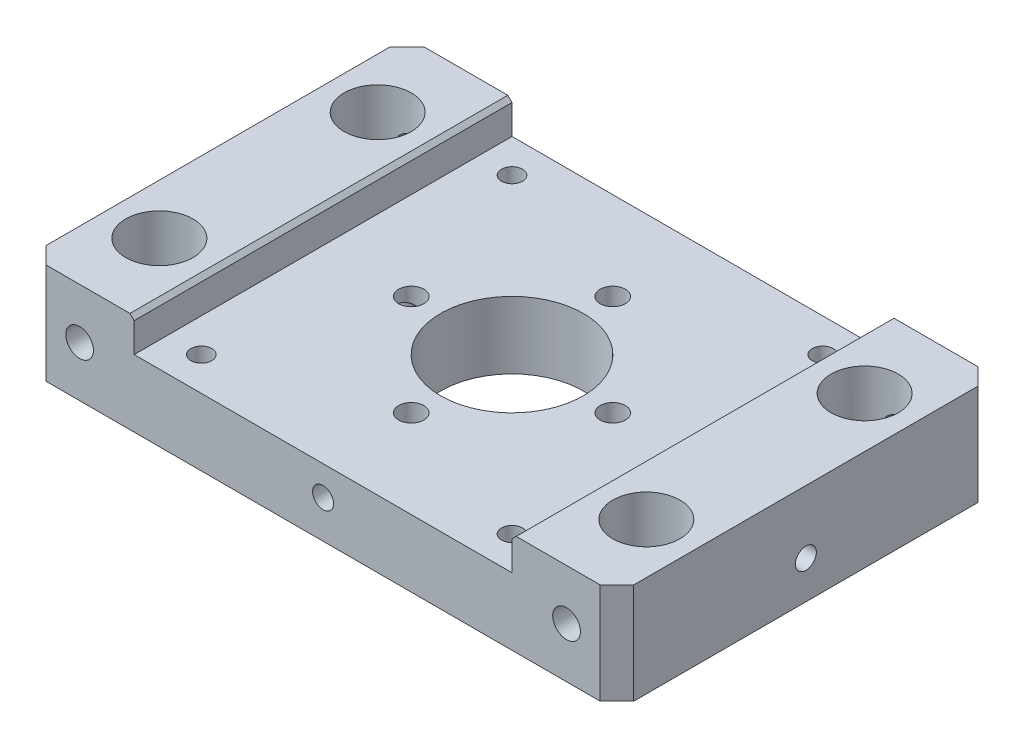
SolidWorks part; units mm, degrees
ref_plane "Front Plane" through (0, 0, 0) normal (0, 0, 1) x (1, 0, 0)
ref_plane "Top Plane" through (0, 0, 0) normal (0, 1, 0) x (1, 0, 0)
ref_plane "Right Plane" through (0, 0, 0) normal (1, 0, 0) x (0, 0, -1)
sketch "Sketch1" plane through (0, 0, 0) normal (0, 1, 0) x (1, 0, 0)
  line L1 (-35, 22.5) -> (35, 22.5)
  line L2 (-35, 22.5) -> (-35, -22.5)
  line L3 (-35, -22.5) -> (35, -22.5)
  line L4 (35, 22.5) -> (35, -22.5)
  line L5 (-35, 22.5) -> (35, -22.5) construction
  line L6 (-35, -22.5) -> (35, 22.5) construction
  point P0 (0, 0)
  dimension "D1" = 45
  dimension "D2" = 70
extrude "Boss-Extrude1" add sketch "Sketch1" along normal blind 12
sketch "Sketch2" plane through (0, 12, 0) normal (0, 1, 0) x (1, 0, 0)
  line L0 (35, 22.5) -> (-35, 22.5) construction
  line L1 (-22.5, -22.5) -> (22.5, -22.5)
  line L2 (-22.5, -22.5) -> (-22.5, 22.5)
  line L3 (-22.5, 22.5) -> (22.5, 22.5)
  line L4 (22.5, -22.5) -> (22.5, 22.5)
  line L5 (-22.5, -22.5) -> (22.5, 22.5) construction
  line L6 (-22.5, 22.5) -> (22.5, -22.5) construction
  point P0 (0, 0)
  dimension "D1" = 45
extrude "Cut-Extrude1" cut sketch "Sketch2" against normal blind 4
sketch "Sketch3" plane through (0, 12, 0) normal (0, 1, 0) x (1, 0, 0)
  line L0 (0, 0) -> (50000, 0) construction
  line L1 (0, 0) -> (0, -50000) construction
  circle A0 centre (-29, 13) radius 4
  circle A1 centre (-29, -13) radius 4
  circle A2 centre (29, -13) radius 4
  circle A3 centre (29, 13) radius 4
  dimension "D2" = 26
  dimension "D3" = 8
  dimension "D1" = 58
extrude "Cut-Extrude2" cut sketch "Sketch3" against normal blind 50
sketch "Sketch4" plane through (0, 12, 0) normal (0, 1, 0) x (1, 0, 0)
  circle A0 centre (0, 0) radius 8.5
  dimension "D1" = 17
extrude "Cut-Extrude3" cut sketch "Sketch4" against normal blind 50
sketch "Sketch5" plane through (0, 0, 22.5) normal (0, 0, 1) x (1, 0, 0)
  line L0 (0, 0) -> (0, -50000) construction
  line L1 (-35, 6) -> (49965, 6) construction
  line L2 (-35, 12) -> (-35, 0) construction
  line L3 (-29, 0) -> (-29, 50000) construction
  line L4 (-35, 12) -> (-22.5, 12) construction
  line L8 (-25, 0) -> (-25, 12) construction
  line L9 (-33, 12) -> (-33, 0) construction
  circle A0 centre (-29, 6) radius 0.5
  circle A1 centre (29, 6) radius 0.5
  point P7 (-35, 6)
  dimension "D1" = 1
extrude "Cut-Extrude4" cut sketch "Sketch5" against normal blind 7
hole_wizard "M4 Tapped Hole1" positions "3DSketch1" profile "Sketch6" tap size "M4" standard "Gb"
sketch3d "3DSketch1"
  line L0 (-29, 6, 17) -> (-29, 6, 22.5) construction
  line L1 (29, 6, 17) -> (29, 6, 22.5) construction
  point P0 (-29, 6, 22.5)
  point P4 (29, 6, 22.5)
sketch "Sketch6" plane through (-29, 6, 22.5) normal (1, 0, 0) x (0, -1, 0)
  line L0 (0, 0) -> (0, 11.0914)
  line L1 (0, 11.0914) -> (1.65, 10.1)
  line L2 (1.65, 10.1) -> (1.65, 0)
  line L5 (1.65, 0) -> (0, 0)
  line L10 (0, 11.0914) -> (-1.65, 10.1) construction
  line L11 (0, -6.35) -> (0, 107.95) construction
  dimension "螺纹孔钻头直径" = 3.3
  dimension "螺纹孔钻头深度" = 10.1
  dimension "导头角度" = 118
cosmetic thread "Hole thread1" parameters "D1"=5.8562, "D2"=4
cosmetic thread "Hole thread2" parameters "D1"=5.8562, "D2"=4
mirror "Mirror1" about plane through (0, 0, 0) normal (0, 0, 1) of "M4 Tapped Hole1"
sketch "Sketch7" plane through (0, 8, 0) normal (0, 1, 0) x (1, 0, 0)
  line L0 (0, 0) -> (50000, 0) construction
  line L1 (0, 0) -> (0, -50000) construction
  circle A0 centre (0, 0) radius 12 construction
  circle A1 centre (0, 12) radius 1.5
  circle A2 centre (12, 0) radius 1.5
  circle A3 centre (0, -12) radius 1.5
  circle A4 centre (-12, 0) radius 1.5
  dimension "D1" = 24
  dimension "D2" = 3
extrude "Cut-Extrude5" cut sketch "Sketch7" against normal blind 4.8
sketch "Sketch8" plane through (-35, 0, 0) normal (-1, 0, 0) x (0, 0, 1)
  line L0 (0, 0) -> (0, 50000) construction
  line L1 (-22.5, 0) -> (22.5, 0) construction
  circle A0 centre (0, 4.5) radius 1.25
  dimension "D1" = 2.5
  dimension "D2" = 4.5
extrude "Cut-Extrude6" cut sketch "Sketch8" against normal blind 23
cosmetic thread "Hole thread9" parameters "D1"=6, "D2"=3
pattern_circular "CirPattern1" count 4 over 360 about axis through (0, -38, 0) along (0, 1, 0) of "Cut-Extrude6"
cosmetic thread "Hole thread7" parameters "D1"=6, "D2"=3
cosmetic thread "Hole thread8" parameters "D1"=6, "D2"=3
cosmetic thread "Hole thread10" parameters "D1"=6, "D2"=3
cosmetic thread "Hole thread11" parameters "D1"=6, "D2"=3
hole_wizard "M3 Tapped Hole4" positions "3DSketch2" profile "Sketch9" tap size "M3" standard "Gb"
sketch3d "3DSketch2"
  line L2 (12.8292, 4.5, 0) -> (35, 4.5, 0) construction
  point P8 (35, 4.5, 0)
sketch "Sketch9" plane through (35, 4.5, 0) normal (0, 1, 0) x (0, 0, -1)
  line L0 (0, 0) -> (0, 6.7511)
  line L1 (0, 6.7511) -> (1.25, 6)
  line L2 (1.25, 6) -> (1.25, 0)
  line L5 (1.25, 0) -> (0, 0)
  line L10 (0, 6.7511) -> (-1.25, 6) construction
  line L11 (0, -6.35) -> (0, 107.95) construction
  dimension "螺纹孔钻头直径" = 2.5
  dimension "螺纹孔钻头深度" = 6
  dimension "导头角度" = 118
cosmetic thread "Hole thread4" parameters "D1"=6, "D2"=3
hole_wizard "M3 Tapped Hole3" positions "3DSketch3" profile "Sketch10" tap size "M3" standard "Gb"
sketch3d "3DSketch3"
  line L1 (0, 4.5, 13.5) -> (0, 4.5, 22.5) construction
  line L2 (0, 4.5, -12.8292) -> (0, 4.5, -22.5) construction
  point P4 (0, 4.5, 22.5)
  point P8 (0, 4.5, -22.5)
sketch "Sketch10" plane through (0, 4.5, 22.5) normal (1, 0, 0) x (0, -1, 0)
  line L0 (0, 0) -> (0, 8.2511)
  line L1 (0, 8.2511) -> (1.25, 7.5)
  line L2 (1.25, 7.5) -> (1.25, 0)
  line L5 (1.25, 0) -> (0, 0)
  line L10 (0, 8.2511) -> (-1.25, 7.5) construction
  line L11 (0, -6.35) -> (0, 107.95) construction
  dimension "螺纹孔钻头直径" = 2.5
  dimension "螺纹孔钻头深度" = 7.5
  dimension "导头角度" = 118
sketch "Sketch11" plane through (35, 0, 0) normal (1, 0, 0) x (0, 0, -1)
  circle A0 centre (0, 4.5) radius 1.25
  dimension "D1" = 2.5
extrude "Cut-Extrude7" [suppressed] cut sketch "Sketch11" against normal up to next
chamfer "Chamfer1" distance 0.5 angle 45 2 edges at (22.5, 12, 0) (-22.5, 12, 0)
hole_wizard "M5 Tapped Hole1" positions "3DSketch4" profile "Sketch12" tap size "M5" standard "Gb"
sketch3d "3DSketch4"
  line L0 (-12.8292, 4.5, 0) -> (-35, 4.5, 0) construction
  point P0 (-35, 4.5, 0)
sketch "Sketch12" plane through (-35, 4.5, 0) normal (0, 1, 0) x (0, 0, 1)
  line L0 (0, 0) -> (0, 11.6618)
  line L1 (0, 11.6618) -> (2.1, 10.4)
  line L2 (2.1, 10.4) -> (2.1, 0)
  line L5 (2.1, 0) -> (0, 0)
  line L10 (0, 11.6618) -> (-2.1, 10.4) construction
  line L11 (0, -6.35) -> (0, 107.95) construction
  dimension "螺纹孔钻头直径" = 4.2
  dimension "螺纹孔钻头深度" = 10.4
  dimension "导头角度" = 118
cosmetic thread "Hole thread12" parameters "D1"=8, "D2"=5
sketch "Sketch13" plane through (-35, 0, 0) normal (-1, 0, 0) x (0, 0, 1)
  circle A0 centre (0, 4.5) radius 2
  dimension "D1" = 4
extrude "Cut-Extrude8" cut sketch "Sketch13" against normal blind 24.5
chamfer "Chamfer2" distance 2 angle 45 4 edges at (35, 6, -22.5) (35, 6, 22.5) (-35, 6, 22.5) (-35, 6, -22.5)
hole_wizard "M3 Tapped Hole5" positions "Sketch15" profile "Sketch14" tap size "M3" standard "Gb" end condition through all
sketch "Sketch15" plane through (0, 8, 0) normal (0, 1, 0) x (1, 0, 0)
  point P0 (18.5, 18.5)
  point P2 (-18.5, 18.5)
  point P5 (-18.5, -18.5)
  point P8 (18.5, -18.5)
sketch "Sketch14" plane through (18.5, 8, -18.5) normal (1, 0, 0) x (0, 0, 1)
  line L0 (0, 0) -> (0, 8)
  line L1 (0, 8) -> (1.25, 8)
  line L2 (1.25, 8) -> (1.25, 0)
  line L5 (1.25, 0) -> (0, 0)
  line L11 (0, -6.35) -> (0, 107.95) construction
  dimension "通孔螺纹孔钻头直径" = 2.5
  dimension "通孔螺纹孔钻头深度" = 8
cosmetic thread "Hole thread13" parameters "D2"=3
cosmetic thread "Hole thread14" parameters "D2"=3
cosmetic thread "Hole thread15" parameters "D2"=3
cosmetic thread "Hole thread16" parameters "D2"=3
hole_wizard "M3 Tapped Hole6" positions "Sketch17" profile "Sketch16" tap size "M3" standard "Gb"
sketch "Sketch17" plane through (0, 0, -22.5) normal (0, 0, -1) x (-1, 0, 0)
  line L0 (-33, 0) -> (33, 0) construction
  point P0 (11.5, 5.5)
  dimension "D1" = 5.5
  dimension "D2" = 11.5
sketch "Sketch16" plane through (-11.5, 5.5, -22.5) normal (1, 0, 0) x (0, 1, 0)
  line L0 (0, 0) -> (0, 8.2511)
  line L1 (0, 8.2511) -> (1.25, 7.5)
  line L2 (1.25, 7.5) -> (1.25, 0)
  line L5 (1.25, 0) -> (0, 0)
  line L10 (0, 8.2511) -> (-1.25, 7.5) construction
  line L11 (0, -6.35) -> (0, 107.95) construction
  dimension "螺纹孔钻头直径" = 2.5
  dimension "螺纹孔钻头深度" = 7.5
  dimension "导头角度" = 118
cosmetic thread "Hole thread17" parameters "D1"=6, "D2"=3
